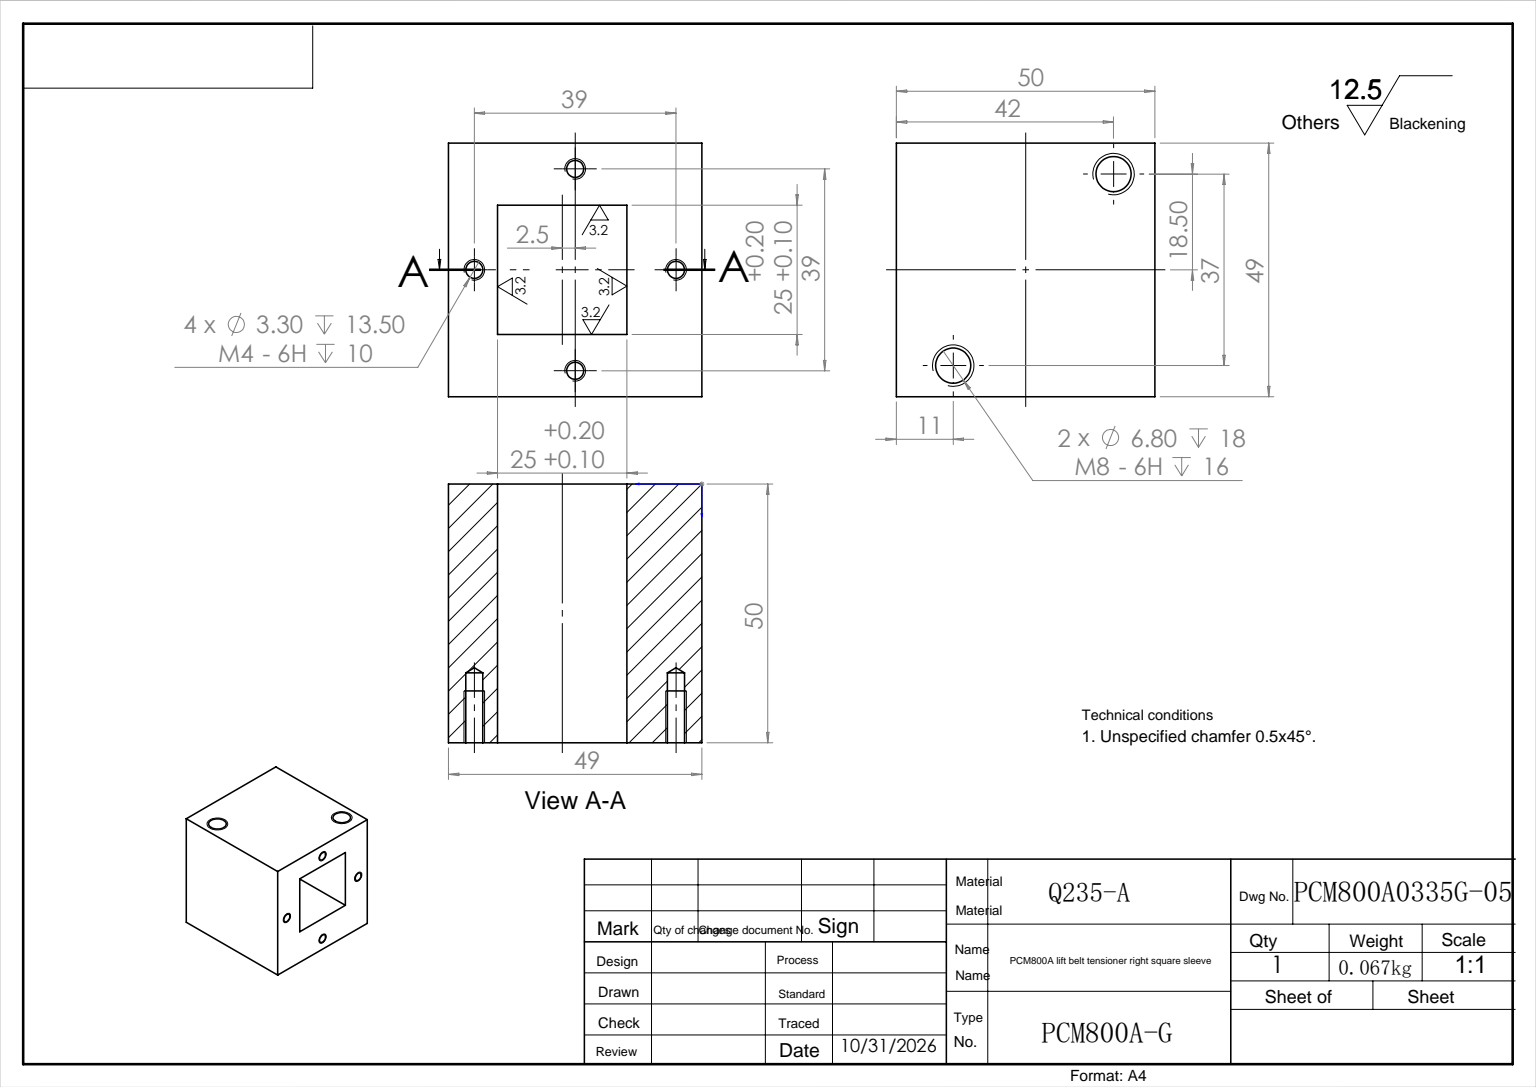
from build123d import *

# Parameters (mm, degrees)
SKETCH_2_W             = 49
SKETCH_2_H             = 49
EXTRUDE_2_DEPTH        = 50
SKETCH_3_W             = 25
SKETCH_3_H             = 25
CUT_EXTRUDE_1_DEPTH    = 50
HOLE_WIZARD_M4_1_D     = 3.3
HOLE_WIZARD_M4_1_DEPTH = 13.5
HOLE_WIZARD_M4_1_TIP   = 0.991420021
HOLE_WIZARD_M8_1_D     = 6.8
HOLE_WIZARD_M8_1_DEPTH = 18
HOLE_WIZARD_M8_1_TIP   = 2.042926105


with BuildPart() as part:
    # 草图2 → 凸台-拉伸2 (new body)
    with BuildSketch(Plane(origin=(0, 0, 0), x_dir=(0, 0, -1), z_dir=(1, 0, 0))):
        with Locations((24.5, 24.5)):
            Rectangle(SKETCH_2_W, SKETCH_2_H)
    extrude(amount=EXTRUDE_2_DEPTH)

    # 草图3 → 切除-拉伸1 (cut)
    with BuildSketch(Plane(origin=(50, 0, 0), x_dir=(0, 0, -1), z_dir=(1, 0, 0))):
        with Locations((24.5, 27)):
            Rectangle(SKETCH_3_W, SKETCH_3_H)
    extrude(amount=-CUT_EXTRUDE_1_DEPTH, mode=Mode.SUBTRACT)

    # M4 螺纹孔1
    with Locations(Plane(origin=(50, 0, 0), x_dir=(0, 0, -1), z_dir=(1, 0, 0))):
        with Locations((24.5, 44), (5, 24.5), (24.5, 5), (44, 24.5)):
            Hole(HOLE_WIZARD_M4_1_D / 2, depth=HOLE_WIZARD_M4_1_DEPTH)
            with Locations((0, 0, -(HOLE_WIZARD_M4_1_DEPTH + HOLE_WIZARD_M4_1_TIP / 2))):  # 118° drill point
                Cone(0, HOLE_WIZARD_M4_1_D / 2, HOLE_WIZARD_M4_1_TIP, mode=Mode.SUBTRACT)

    # M8 螺纹孔1
    with Locations(Plane(origin=(0, 49, 0), x_dir=(-1, 0, 0), z_dir=(0, 1, 0))):
        with Locations((-11, -6), (-42, -43)):
            Hole(HOLE_WIZARD_M8_1_D / 2, depth=HOLE_WIZARD_M8_1_DEPTH)
            with Locations((0, 0, -(HOLE_WIZARD_M8_1_DEPTH + HOLE_WIZARD_M8_1_TIP / 2))):  # 118° drill point
                Cone(0, HOLE_WIZARD_M8_1_D / 2, HOLE_WIZARD_M8_1_TIP, mode=Mode.SUBTRACT)


solid = part.part
